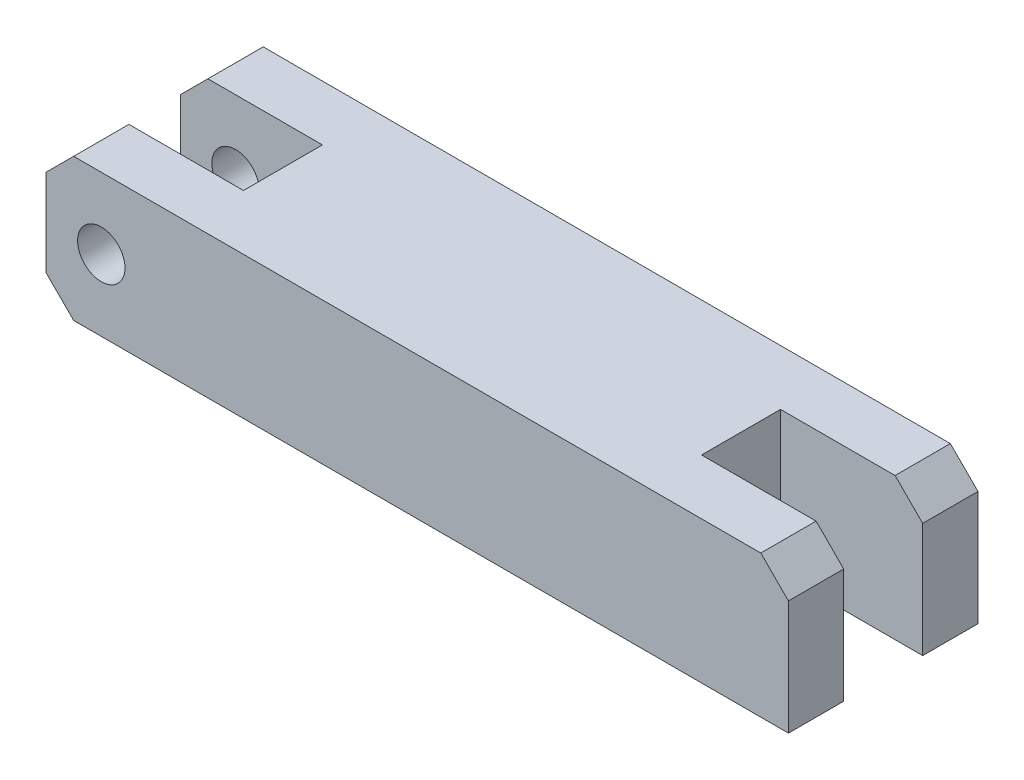
SolidWorks part; units mm, degrees
material "S45C"
ref_plane "Front Plane" through (0, 0, 0) normal (0, 0, 1) x (1, 0, 0)
ref_plane "Top Plane" through (0, 0, 0) normal (0, 1, 0) x (1, 0, 0)
ref_plane "Right Plane" through (0, 0, 0) normal (1, 0, 0) x (0, 0, -1)
sketch "Sketch1" plane through (0, 0, 0) normal (0, 1, 0) x (1, 0, 0)
  line L1 (-47, 12) -> (47, 12)
  line L2 (-47, 12) -> (-47, -12)
  line L3 (-47, -12) -> (47, -12)
  line L4 (47, 12) -> (47, -12)
  line L5 (-47, 12) -> (47, -12) construction
  line L6 (-47, -12) -> (47, 12) construction
  point P0 (0, 0)
  dimension "D1" = 94
  dimension "D2" = 24
extrude "Boss-Extrude1" add sketch "Sketch1" along normal blind 18
sketch "Sketch2" plane through (0, 18, 0) normal (0, 1, 0) x (1, 0, 0)
  line L0 (-47, 12) -> (-47, -12) construction
  line L1 (-65, 5) -> (-29, 5)
  line L2 (-65, 5) -> (-65, -5)
  line L3 (-65, -5) -> (-29, -5)
  line L4 (-29, 5) -> (-29, -5)
  line L5 (-65, 5) -> (-29, -5) construction
  line L6 (-65, -5) -> (-29, 5) construction
  line L7 (0, 0) -> (0, 22.1272) construction
  line L8 (65, -5) -> (29, 5) construction
  line L9 (65, 5) -> (29, -5) construction
  line L10 (29, 5) -> (29, -5)
  line L11 (65, -5) -> (29, -5)
  line L12 (65, 5) -> (65, -5)
  line L13 (65, 5) -> (29, 5)
  point P0 (-47, 0)
  point P14 (47, 0)
  dimension "D1" = 36
  dimension "D2" = 10
extrude "Cut-Extrude1" cut sketch "Sketch2" against normal blind 70
chamfer "Chamfer1" distance 3.5 angle 45 2 edges at (47, 18, 8.5) (47, 18, -8.5)
chamfer "Chamfer2" distance 3.5 angle 45 4 edges at (-47, 0, 8.5) (-47, 0, -8.5) (-47, 18, -8.5) (-47, 18, 8.5)
sketch "Sketch3" plane through (0, 0, 12) normal (0, 0, 1) x (1, 0, 0)
  line L0 (-43.5, 0) -> (47, 0) construction
  line L1 (-47, 14.5) -> (-47, 3.5) construction
  circle A0 centre (-40, 9) radius 3
  dimension "D3" = 6
  dimension "D1" = 9
  dimension "D2" = 7
extrude "Cut-Extrude2" cut sketch "Sketch3" against normal blind 70
